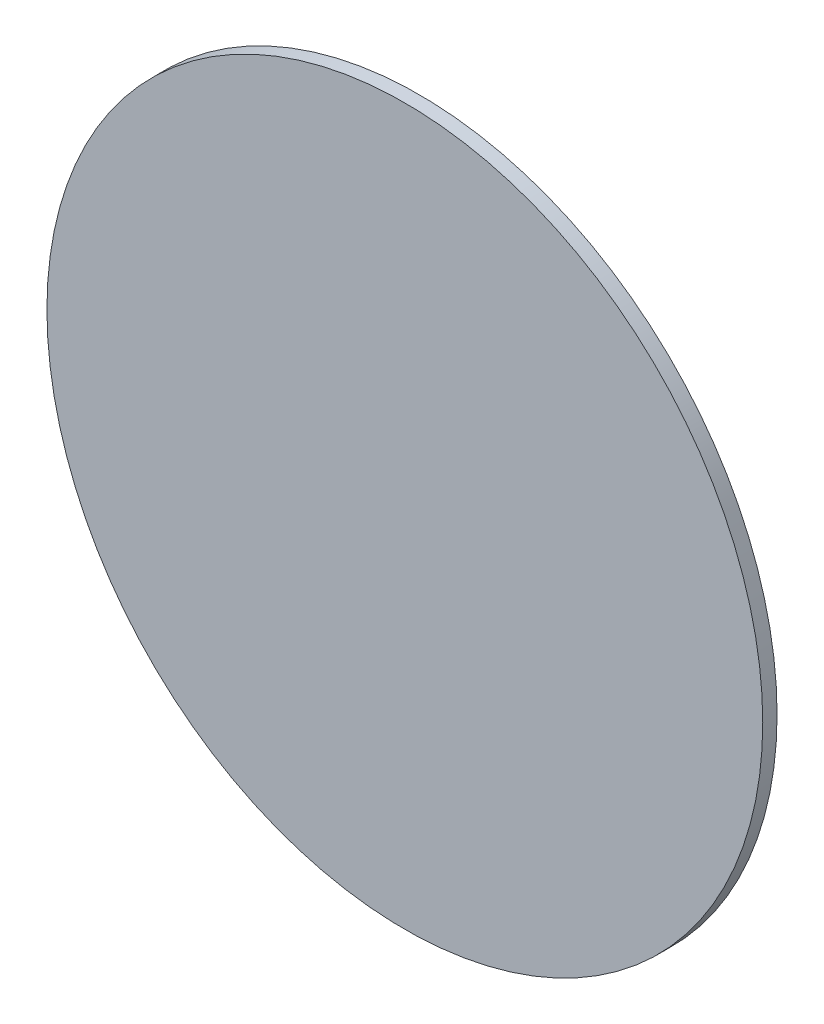
SolidWorks part; units mm, degrees
material "玻璃"
ref_plane "Front" through (0, 0, 0) normal (0, 0, 1) x (1, 0, 0)
ref_plane "Top" through (0, 0, 0) normal (0, 1, 0) x (1, 0, 0)
ref_plane "Right" through (0, 0, 0) normal (1, 0, 0) x (0, 0, -1)
sketch "草图1" plane through (0, 0, 0) normal (0, 0, 1) x (1, 0, 0)
  circle A0 centre (0, 0) radius 25
  dimension "D1" = 50
extrude "凸台-拉伸1" add sketch "草图1" along normal mid plane 1
